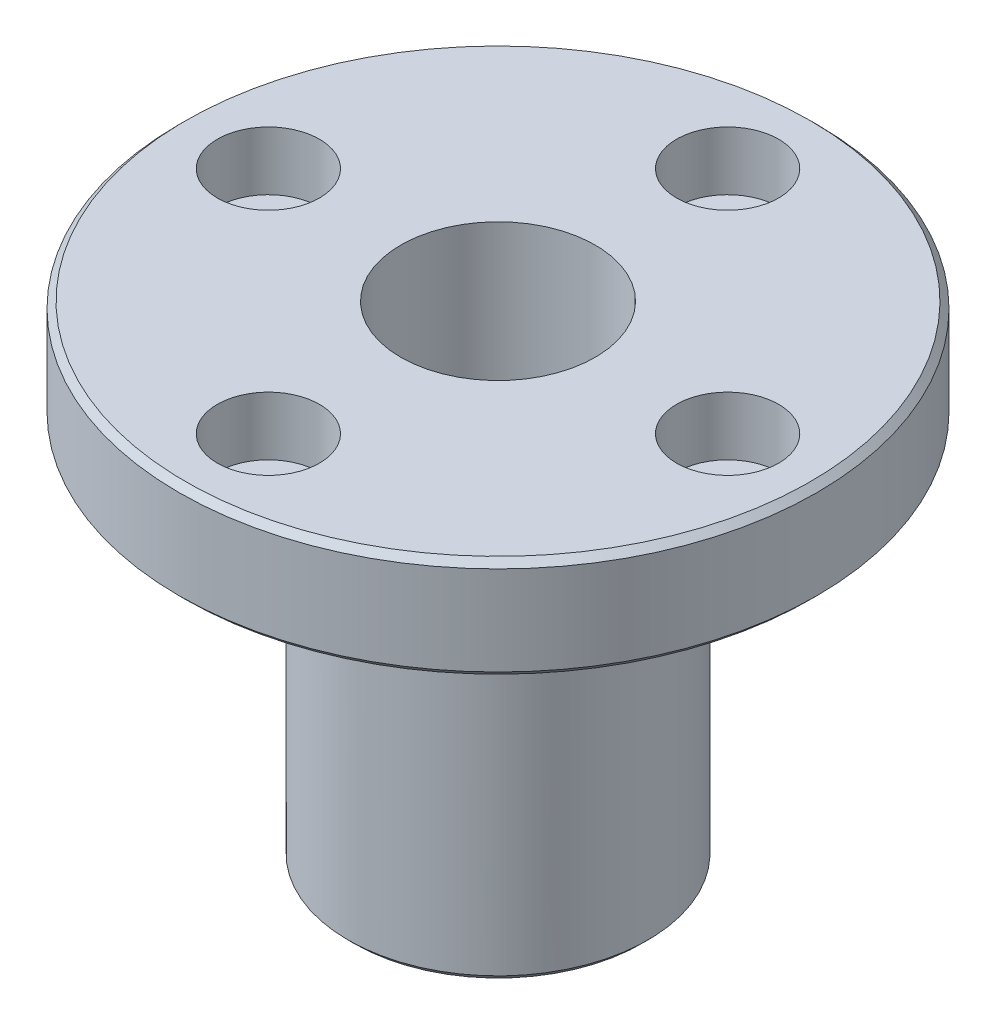
SolidWorks part; units mm, degrees
material "AISI Type 316L Stainless Steel"
ref_plane "Front Plane" through (0, 0, 0) normal (0, 0, 1) x (1, 0, 0)
ref_plane "Top Plane" through (0, 0, 0) normal (0, 1, 0) x (1, 0, 0)
ref_plane "Right Plane" through (0, 0, 0) normal (1, 0, 0) x (0, 0, -1)
sketch "Sketch1" plane through (0, 0, 0) normal (0, 0, 1) x (1, 0, 0)
  line L0 (0, 0) -> (0, 38) construction
  line L1 (0, 38) -> (-25, 38)
  line L2 (-25, 38) -> (-25, 30)
  line L3 (-25, 30) -> (-11.75, 30)
  line L4 (-11.75, 30) -> (-11.75, 0)
  line L5 (-11.75, 0) -> (0, 0)
  line L6 (0, 0) -> (0, 38)
  dimension "D1" = 23.5
  dimension "D2" = 50
  dimension "D3" = 8
  dimension "D4" = 38
revolve "Revolve1" add sketch "Sketch1" angle 360 about L0
sketch "Sketch3" plane through (0, 38, 0) normal (0, 1, 0) x (1, 0, 0)
  point P0 (0, 0)
hole_wizard "G1/4 Tapped Hole1" positions "3DSketch1" profile "Sketch4" tap size "G1/4" standard "GB"
sketch3d "3DSketch1"
  point P0 (0, 30, 0)
sketch "Sketch4" plane through (0, 30, 0) normal (1, 0, 0) x (0, 0, 1)
  line L0 (0, 0) -> (0, 30)
  line L1 (0, 30) -> (5.9, 30)
  line L2 (5.9, 30) -> (5.9, 0)
  line L5 (5.9, 0) -> (0, 0)
  line L11 (0, -6.35) -> (0, 107.95) construction
  dimension "通孔螺纹孔钻头直径" = 11.8
  dimension "通孔螺纹孔钻头深度" = 30
cosmetic thread "Cosmetic Thread1" [suppressed] parameters "D2"=13.157
hole_wizard "G3/8 Tapped Hole1" positions "3DSketch2" profile "Sketch5" tap size "G3/8" standard "GB" end condition through all
sketch3d "3DSketch2"
  point P0 (0, 38, 0)
cosmetic thread "Cosmetic Thread2"
sketch "Sketch5" plane through (0, 38, 0) normal (1, 0, 0) x (0, 0, 1)
  line L0 (0, 0) -> (0, 38)
  line L1 (0, 38) -> (7.625, 38)
  line L2 (7.625, 38) -> (7.625, 0)
  line L5 (7.625, 0) -> (0, 0)
  line L11 (0, -6.35) -> (0, 107.95) construction
  dimension "通孔螺纹孔钻头直径" = 15.25
  dimension "通孔螺纹孔钻头深度" = 38
sketch "Sketch6" plane through (0, 38, 0) normal (0, 1, 0) x (1, 0, 0)
  line L0 (0, 18) -> (0, -18) construction
  line L1 (-18, 0) -> (18, 0) construction
  circle A0 centre (0, 0) radius 18 construction
  dimension "D1" = 36
hole_wizard "Hole Size (per socket head cap screw type)1" positions "3DSketch3" profile "Sketch7" counterbore size "M4" standard "GB" end condition through all
sketch3d "3DSketch3"
  point P0 (0, 38, -18)
  point P3 (-18, 38, 0)
  point P6 (18, 38, 0)
  point P9 (0, 38, 18)
sketch "Sketch7" plane through (0, 38, -18) normal (1, 0, 0) x (0, 0, 1)
  line L0 (0, 0) -> (0, 38)
  line L1 (0, 38) -> (2.25, 38)
  line L3 (2.25, 38) -> (2.25, 4.6)
  line L4 (2.25, 4.6) -> (4, 4.6)
  line L5 (4, 4.6) -> (4, 0)
  line L7 (4, 0) -> (0, 0)
  line L11 (0, -6.35) -> (0, 107.95) construction
  dimension "通孔孔直径" = 4.5
  dimension "通孔孔深度" = 38
  dimension "柱形沉头孔直径" = 8
  dimension "柱形沉头孔深度" = 4.6
chamfer "Chamfer1" distance 0.5 angle 45 3 edges at (0, 0, -11.75) (0, 30, -25) (0, 38, -25)
